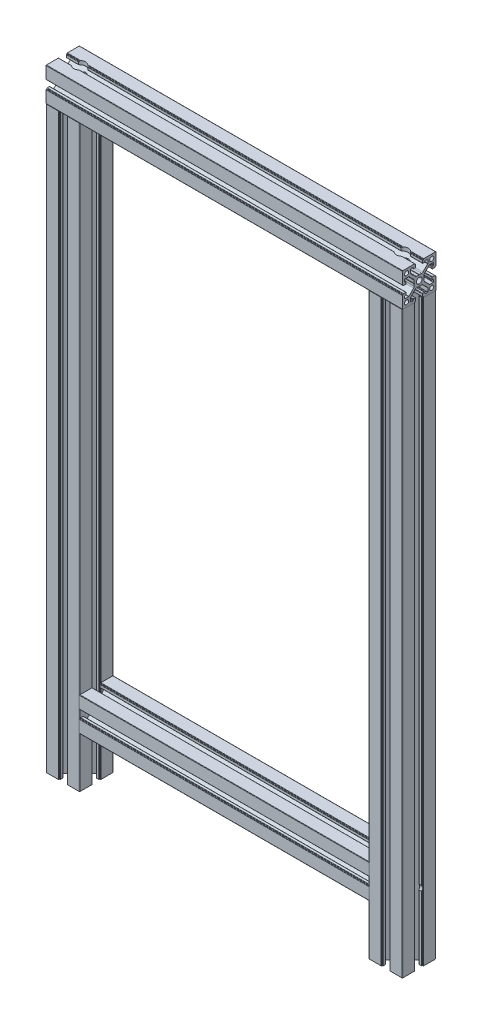
from build123d import *

# Parameters (mm, degrees)
SKETCH_14_R                = 2.45
SKETCH_14_R_2              = 3.4
LE_8_4040HW_DEPTH          = 425
SKETCH_14_ON_SEGMENT_2_R   = 2.45
SKETCH_14_ON_SEGMENT_2_R_2 = 3.4
LE_8_4040HW_2_DEPTH        = 711.5
SKETCH_14_ON_SEGMENT_3_R   = 2.45
SKETCH_14_ON_SEGMENT_3_R_2 = 3.4
LE_8_4040HW_3_DEPTH        = 711.5
SKETCH_14_ON_SEGMENT_4_R   = 2.45
SKETCH_14_ON_SEGMENT_4_R_2 = 3.4
LE_8_4040HW_4_DEPTH        = 387
SKETCH_15_R                = 4.4
CUT_EXTRUDE_1_DEPTH        = 46
SKETCH_16_R                = 5.1
CUT_EXTRUDE_3_DEPTH        = 40
SKETCH_18_R                = 7
CUT_EXTRUDE_8_DEPTH        = 30


with BuildPart() as part:
    # 草图14 → LE-8-4040HW (new body)
    with BuildSketch(Plane(origin=(-212.5, 710.5, 0), x_dir=(0, 1, 0), z_dir=(1, 0, 0))):
        with BuildLine():
            Line((-6, -0.3), (-6, -3.050252532))
            ThreePointArc((-6, -3.050252532), (-6.152240935, -3.815619396), (-6.585786438, -4.464466094))
            Line((-6.585786438, -4.464466094), (-12.224873734, -10.103553391))
            ThreePointArc((-12.224873734, -10.103553391), (-12.387085409, -10.211939766), (-12.578427125, -10.25))
            Line((-12.578427125, -10.25), (-16.8, -10.25))
            ThreePointArc((-16.8, -10.25), (-17.153553391, -10.103553391), (-17.3, -9.75))
            Line((-17.3, -9.75), (-17.3, -7.6))
            ThreePointArc((-17.3, -7.6), (-17.153553391, -7.246446609), (-16.8, -7.1))
            Line((-16.8, -7.1), (-16, -7.1))
            ThreePointArc((-16, -7.1), (-15.646446609, -6.953553391), (-15.5, -6.6))
            Line((-15.5, -6.6), (-15.5, -4.6))
            ThreePointArc((-15.5, -4.6), (-15.646446609, -4.246446609), (-16, -4.1))
            Line((-16, -4.1), (-18.7, -4.1))
            ThreePointArc((-18.7, -4.1), (-18.912132034, -4.187867966), (-19, -4.4))
            Line((-19, -4.4), (-19, -4.8))
            ThreePointArc((-19, -4.8), (-19.087867966, -5.012132034), (-19.3, -5.1))
            Line((-19.3, -5.1), (-19.7, -5.1))
            ThreePointArc((-19.7, -5.1), (-19.912132034, -5.187867966), (-20, -5.4))
            Line((-20, -5.4), (-20, -19.5))
            ThreePointArc((-20, -19.5), (-19.853553391, -19.853553391), (-19.5, -20))
            Line((-19.5, -20), (-5.4, -20))
            ThreePointArc((-5.4, -20), (-5.187867966, -19.912132034), (-5.1, -19.7))
            Line((-5.1, -19.7), (-5.1, -19.3))
            ThreePointArc((-5.1, -19.3), (-5.012132034, -19.087867966), (-4.8, -19))
            Line((-4.8, -19), (-4.4, -19))
            ThreePointArc((-4.4, -19), (-4.187867966, -18.912132034), (-4.1, -18.7))
            Line((-4.1, -18.7), (-4.1, -16))
            ThreePointArc((-4.1, -16), (-4.246446609, -15.646446609), (-4.6, -15.5))
            Line((-4.6, -15.5), (-6.6, -15.5))
            ThreePointArc((-6.6, -15.5), (-6.953553391, -15.646446609), (-7.1, -16))
            Line((-7.1, -16), (-7.1, -16.8))
            ThreePointArc((-7.1, -16.8), (-7.246446609, -17.153553391), (-7.6, -17.3))
            Line((-7.6, -17.3), (-9.75, -17.3))
            ThreePointArc((-9.75, -17.3), (-10.103553391, -17.153553391), (-10.25, -16.8))
            Line((-10.25, -16.8), (-10.25, -12.578427125))
            ThreePointArc((-10.25, -12.578427125), (-10.211939766, -12.387085409), (-10.103553391, -12.224873734))
            Line((-10.103553391, -12.224873734), (-4.464466094, -6.585786438))
            ThreePointArc((-4.464466094, -6.585786438), (-3.815619396, -6.152240935), (-3.050252532, -6))
            Line((-3.050252532, -6), (-0.3, -6))
            ThreePointArc((-0.3, -6), (0, -5.7), (0.3, -6))
            Line((0.3, -6), (3.050252532, -6))
            ThreePointArc((3.050252532, -6), (3.815619396, -6.152240935), (4.464466094, -6.585786438))
            Line((4.464466094, -6.585786438), (10.103553391, -12.224873734))
            ThreePointArc((10.103553391, -12.224873734), (10.211939766, -12.387085409), (10.25, -12.578427125))
            Line((10.25, -12.578427125), (10.25, -16.8))
            ThreePointArc((10.25, -16.8), (10.103553391, -17.153553391), (9.75, -17.3))
            Line((9.75, -17.3), (7.6, -17.3))
            ThreePointArc((7.6, -17.3), (7.246446609, -17.153553391), (7.1, -16.8))
            Line((7.1, -16.8), (7.1, -16))
            ThreePointArc((7.1, -16), (6.953553391, -15.646446609), (6.6, -15.5))
            Line((6.6, -15.5), (4.6, -15.5))
            ThreePointArc((4.6, -15.5), (4.246446609, -15.646446609), (4.1, -16))
            Line((4.1, -16), (4.1, -18.7))
            ThreePointArc((4.1, -18.7), (4.187867966, -18.912132034), (4.4, -19))
            Line((4.4, -19), (4.8, -19))
            ThreePointArc((4.8, -19), (5.012132034, -19.087867966), (5.1, -19.3))
            Line((5.1, -19.3), (5.1, -19.7))
            ThreePointArc((5.1, -19.7), (5.187867966, -19.912132034), (5.4, -20))
            Line((5.4, -20), (19.5, -20))
            ThreePointArc((19.5, -20), (19.853553391, -19.853553391), (20, -19.5))
            Line((20, -19.5), (20, -5.4))
            ThreePointArc((20, -5.4), (19.912132034, -5.187867966), (19.7, -5.1))
            Line((19.7, -5.1), (19.3, -5.1))
            ThreePointArc((19.3, -5.1), (19.087867966, -5.012132034), (19, -4.8))
            Line((19, -4.8), (19, -4.4))
            ThreePointArc((19, -4.4), (18.912132034, -4.187867966), (18.7, -4.1))
            Line((18.7, -4.1), (16, -4.1))
            ThreePointArc((16, -4.1), (15.646446609, -4.246446609), (15.5, -4.6))
            Line((15.5, -4.6), (15.5, -6.6))
            ThreePointArc((15.5, -6.6), (15.646446609, -6.953553391), (16, -7.1))
            Line((16, -7.1), (16.8, -7.1))
            ThreePointArc((16.8, -7.1), (17.153553391, -7.246446609), (17.3, -7.6))
            Line((17.3, -7.6), (17.3, -9.75))
            ThreePointArc((17.3, -9.75), (17.153553391, -10.103553391), (16.8, -10.25))
            Line((16.8, -10.25), (12.578427125, -10.25))
            ThreePointArc((12.578427125, -10.25), (12.387085409, -10.211939766), (12.224873734, -10.103553391))
            Line((12.224873734, -10.103553391), (6.585786438, -4.464466094))
            ThreePointArc((6.585786438, -4.464466094), (6.152240935, -3.815619396), (6, -3.050252532))
            Line((6, -3.050252532), (6, -0.3))
            ThreePointArc((6, -0.3), (5.7, 0), (6, 0.3))
            Line((6, 0.3), (6, 3.050252532))
            ThreePointArc((6, 3.050252532), (6.152240935, 3.815619396), (6.585786438, 4.464466094))
            Line((6.585786438, 4.464466094), (12.224873734, 10.103553391))
            ThreePointArc((12.224873734, 10.103553391), (12.387085409, 10.211939766), (12.578427125, 10.25))
            Line((12.578427125, 10.25), (16.8, 10.25))
            ThreePointArc((16.8, 10.25), (17.153553391, 10.103553391), (17.3, 9.75))
            Line((17.3, 9.75), (17.3, 7.6))
            ThreePointArc((17.3, 7.6), (17.153553391, 7.246446609), (16.8, 7.1))
            Line((16.8, 7.1), (16, 7.1))
            ThreePointArc((16, 7.1), (15.646446609, 6.953553391), (15.5, 6.6))
            Line((15.5, 6.6), (15.5, 4.6))
            ThreePointArc((15.5, 4.6), (15.646446609, 4.246446609), (16, 4.1))
            Line((16, 4.1), (18.7, 4.1))
            ThreePointArc((18.7, 4.1), (18.912132034, 4.187867966), (19, 4.4))
            Line((19, 4.4), (19, 4.8))
            ThreePointArc((19, 4.8), (19.087867966, 5.012132034), (19.3, 5.1))
            Line((19.3, 5.1), (19.7, 5.1))
            ThreePointArc((19.7, 5.1), (19.912132034, 5.187867966), (20, 5.4))
            Line((20, 5.4), (20, 19.5))
            ThreePointArc((20, 19.5), (19.853553391, 19.853553391), (19.5, 20))
            Line((19.5, 20), (5.4, 20))
            ThreePointArc((5.4, 20), (5.187867966, 19.912132034), (5.1, 19.7))
            Line((5.1, 19.7), (5.1, 19.3))
            ThreePointArc((5.1, 19.3), (5.012132034, 19.087867966), (4.8, 19))
            Line((4.8, 19), (4.4, 19))
            ThreePointArc((4.4, 19), (4.187867966, 18.912132034), (4.1, 18.7))
            Line((4.1, 18.7), (4.1, 16))
            ThreePointArc((4.1, 16), (4.246446609, 15.646446609), (4.6, 15.5))
            Line((4.6, 15.5), (6.6, 15.5))
            ThreePointArc((6.6, 15.5), (6.953553391, 15.646446609), (7.1, 16))
            Line((7.1, 16), (7.1, 16.8))
            ThreePointArc((7.1, 16.8), (7.246446609, 17.153553391), (7.6, 17.3))
            Line((7.6, 17.3), (9.75, 17.3))
            ThreePointArc((9.75, 17.3), (10.103553391, 17.153553391), (10.25, 16.8))
            Line((10.25, 16.8), (10.25, 12.578427125))
            ThreePointArc((10.25, 12.578427125), (10.211939766, 12.387085409), (10.103553391, 12.224873734))
            Line((10.103553391, 12.224873734), (4.464466094, 6.585786438))
            ThreePointArc((4.464466094, 6.585786438), (3.815619396, 6.152240935), (3.050252532, 6))
            Line((3.050252532, 6), (0.3, 6))
            ThreePointArc((0.3, 6), (0, 5.7), (-0.3, 6))
            Line((-0.3, 6), (-3.050252532, 6))
            ThreePointArc((-3.050252532, 6), (-3.815619396, 6.152240935), (-4.464466094, 6.585786438))
            Line((-4.464466094, 6.585786438), (-10.103553391, 12.224873734))
            ThreePointArc((-10.103553391, 12.224873734), (-10.211939766, 12.387085409), (-10.25, 12.578427125))
            Line((-10.25, 12.578427125), (-10.25, 16.8))
            ThreePointArc((-10.25, 16.8), (-10.103553391, 17.153553391), (-9.75, 17.3))
            Line((-9.75, 17.3), (-7.6, 17.3))
            ThreePointArc((-7.6, 17.3), (-7.246446609, 17.153553391), (-7.1, 16.8))
            Line((-7.1, 16.8), (-7.1, 16))
            ThreePointArc((-7.1, 16), (-6.953553391, 15.646446609), (-6.6, 15.5))
            Line((-6.6, 15.5), (-4.6, 15.5))
            ThreePointArc((-4.6, 15.5), (-4.246446609, 15.646446609), (-4.1, 16))
            Line((-4.1, 16), (-4.1, 18.7))
            ThreePointArc((-4.1, 18.7), (-4.187867966, 18.912132034), (-4.4, 19))
            Line((-4.4, 19), (-4.8, 19))
            ThreePointArc((-4.8, 19), (-5.012132034, 19.087867966), (-5.1, 19.3))
            Line((-5.1, 19.3), (-5.1, 19.7))
            ThreePointArc((-5.1, 19.7), (-5.187867966, 19.912132034), (-5.4, 20))
            Line((-5.4, 20), (-19.5, 20))
            ThreePointArc((-19.5, 20), (-19.853553391, 19.853553391), (-20, 19.5))
            Line((-20, 19.5), (-20, 5.4))
            ThreePointArc((-20, 5.4), (-19.912132034, 5.187867966), (-19.7, 5.1))
            Line((-19.7, 5.1), (-19.3, 5.1))
            ThreePointArc((-19.3, 5.1), (-19.087867966, 5.012132034), (-19, 4.8))
            Line((-19, 4.8), (-19, 4.4))
            ThreePointArc((-19, 4.4), (-18.912132034, 4.187867966), (-18.7, 4.1))
            Line((-18.7, 4.1), (-16, 4.1))
            ThreePointArc((-16, 4.1), (-15.646446609, 4.246446609), (-15.5, 4.6))
            Line((-15.5, 4.6), (-15.5, 6.6))
            ThreePointArc((-15.5, 6.6), (-15.646446609, 6.953553391), (-16, 7.1))
            Line((-16, 7.1), (-16.8, 7.1))
            ThreePointArc((-16.8, 7.1), (-17.153553391, 7.246446609), (-17.3, 7.6))
            Line((-17.3, 7.6), (-17.3, 9.75))
            ThreePointArc((-17.3, 9.75), (-17.153553391, 10.103553391), (-16.8, 10.25))
            Line((-16.8, 10.25), (-12.578427125, 10.25))
            ThreePointArc((-12.578427125, 10.25), (-12.387085409, 10.211939766), (-12.224873734, 10.103553391))
            Line((-12.224873734, 10.103553391), (-6.585786438, 4.464466094))
            ThreePointArc((-6.585786438, 4.464466094), (-6.152240935, 3.815619396), (-6, 3.050252532))
            Line((-6, 3.050252532), (-6, 0.3))
            ThreePointArc((-6, 0.3), (-5.7, 0), (-6, -0.3))
        make_face()
        with Locations((-15, 15)):
            Circle(SKETCH_14_R, mode=Mode.SUBTRACT)
        Circle(SKETCH_14_R_2, mode=Mode.SUBTRACT)
        with Locations((15, 15)):
            Circle(SKETCH_14_R, mode=Mode.SUBTRACT)
        with Locations((15, -15)):
            Circle(SKETCH_14_R, mode=Mode.SUBTRACT)
        with Locations((-15, -15)):
            Circle(SKETCH_14_R, mode=Mode.SUBTRACT)
    extrude(amount=LE_8_4040HW_DEPTH)

    # 草图18 → 切除-拉伸8 (cut)
    with BuildSketch(Plane(origin=(0, 730.5, 0), x_dir=(1, 0, 0), z_dir=(0, 1, 0))):
        with Locations(Location((192.5, 0, 0), (0, 0, 320.373457062))):
            Circle(SKETCH_18_R)
        with Locations(Location((-192.5, 0, 0), (0, 0, 320.373457062))):
            Circle(SKETCH_18_R)
    extrude(amount=-CUT_EXTRUDE_8_DEPTH, mode=Mode.SUBTRACT)


with BuildPart() as body_2:
    # 草图14 on segment 2 (carried to segment 2) → LE-8-4040HW 2 (new body)
    with BuildSketch(Plane(origin=(-192.5, 0, 0), x_dir=(-1, 0, 0), z_dir=(0, 1, 0))):
        with BuildLine():
            Line((-6, -0.3), (-6, -3.050252532))
            ThreePointArc((-6, -3.050252532), (-6.152240935, -3.815619396), (-6.585786438, -4.464466094))
            Line((-6.585786438, -4.464466094), (-12.224873734, -10.103553391))
            ThreePointArc((-12.224873734, -10.103553391), (-12.387085409, -10.211939766), (-12.578427125, -10.25))
            Line((-12.578427125, -10.25), (-16.8, -10.25))
            ThreePointArc((-16.8, -10.25), (-17.153553391, -10.103553391), (-17.3, -9.75))
            Line((-17.3, -9.75), (-17.3, -7.6))
            ThreePointArc((-17.3, -7.6), (-17.153553391, -7.246446609), (-16.8, -7.1))
            Line((-16.8, -7.1), (-16, -7.1))
            ThreePointArc((-16, -7.1), (-15.646446609, -6.953553391), (-15.5, -6.6))
            Line((-15.5, -6.6), (-15.5, -4.6))
            ThreePointArc((-15.5, -4.6), (-15.646446609, -4.246446609), (-16, -4.1))
            Line((-16, -4.1), (-18.7, -4.1))
            ThreePointArc((-18.7, -4.1), (-18.912132034, -4.187867966), (-19, -4.4))
            Line((-19, -4.4), (-19, -4.8))
            ThreePointArc((-19, -4.8), (-19.087867966, -5.012132034), (-19.3, -5.1))
            Line((-19.3, -5.1), (-19.7, -5.1))
            ThreePointArc((-19.7, -5.1), (-19.912132034, -5.187867966), (-20, -5.4))
            Line((-20, -5.4), (-20, -19.5))
            ThreePointArc((-20, -19.5), (-19.853553391, -19.853553391), (-19.5, -20))
            Line((-19.5, -20), (-5.4, -20))
            ThreePointArc((-5.4, -20), (-5.187867966, -19.912132034), (-5.1, -19.7))
            Line((-5.1, -19.7), (-5.1, -19.3))
            ThreePointArc((-5.1, -19.3), (-5.012132034, -19.087867966), (-4.8, -19))
            Line((-4.8, -19), (-4.4, -19))
            ThreePointArc((-4.4, -19), (-4.187867966, -18.912132034), (-4.1, -18.7))
            Line((-4.1, -18.7), (-4.1, -16))
            ThreePointArc((-4.1, -16), (-4.246446609, -15.646446609), (-4.6, -15.5))
            Line((-4.6, -15.5), (-6.6, -15.5))
            ThreePointArc((-6.6, -15.5), (-6.953553391, -15.646446609), (-7.1, -16))
            Line((-7.1, -16), (-7.1, -16.8))
            ThreePointArc((-7.1, -16.8), (-7.246446609, -17.153553391), (-7.6, -17.3))
            Line((-7.6, -17.3), (-9.75, -17.3))
            ThreePointArc((-9.75, -17.3), (-10.103553391, -17.153553391), (-10.25, -16.8))
            Line((-10.25, -16.8), (-10.25, -12.578427125))
            ThreePointArc((-10.25, -12.578427125), (-10.211939766, -12.387085409), (-10.103553391, -12.224873734))
            Line((-10.103553391, -12.224873734), (-4.464466094, -6.585786438))
            ThreePointArc((-4.464466094, -6.585786438), (-3.815619396, -6.152240935), (-3.050252532, -6))
            Line((-3.050252532, -6), (-0.3, -6))
            ThreePointArc((-0.3, -6), (0, -5.7), (0.3, -6))
            Line((0.3, -6), (3.050252532, -6))
            ThreePointArc((3.050252532, -6), (3.815619396, -6.152240935), (4.464466094, -6.585786438))
            Line((4.464466094, -6.585786438), (10.103553391, -12.224873734))
            ThreePointArc((10.103553391, -12.224873734), (10.211939766, -12.387085409), (10.25, -12.578427125))
            Line((10.25, -12.578427125), (10.25, -16.8))
            ThreePointArc((10.25, -16.8), (10.103553391, -17.153553391), (9.75, -17.3))
            Line((9.75, -17.3), (7.6, -17.3))
            ThreePointArc((7.6, -17.3), (7.246446609, -17.153553391), (7.1, -16.8))
            Line((7.1, -16.8), (7.1, -16))
            ThreePointArc((7.1, -16), (6.953553391, -15.646446609), (6.6, -15.5))
            Line((6.6, -15.5), (4.6, -15.5))
            ThreePointArc((4.6, -15.5), (4.246446609, -15.646446609), (4.1, -16))
            Line((4.1, -16), (4.1, -18.7))
            ThreePointArc((4.1, -18.7), (4.187867966, -18.912132034), (4.4, -19))
            Line((4.4, -19), (4.8, -19))
            ThreePointArc((4.8, -19), (5.012132034, -19.087867966), (5.1, -19.3))
            Line((5.1, -19.3), (5.1, -19.7))
            ThreePointArc((5.1, -19.7), (5.187867966, -19.912132034), (5.4, -20))
            Line((5.4, -20), (19.5, -20))
            ThreePointArc((19.5, -20), (19.853553391, -19.853553391), (20, -19.5))
            Line((20, -19.5), (20, -5.4))
            ThreePointArc((20, -5.4), (19.912132034, -5.187867966), (19.7, -5.1))
            Line((19.7, -5.1), (19.3, -5.1))
            ThreePointArc((19.3, -5.1), (19.087867966, -5.012132034), (19, -4.8))
            Line((19, -4.8), (19, -4.4))
            ThreePointArc((19, -4.4), (18.912132034, -4.187867966), (18.7, -4.1))
            Line((18.7, -4.1), (16, -4.1))
            ThreePointArc((16, -4.1), (15.646446609, -4.246446609), (15.5, -4.6))
            Line((15.5, -4.6), (15.5, -6.6))
            ThreePointArc((15.5, -6.6), (15.646446609, -6.953553391), (16, -7.1))
            Line((16, -7.1), (16.8, -7.1))
            ThreePointArc((16.8, -7.1), (17.153553391, -7.246446609), (17.3, -7.6))
            Line((17.3, -7.6), (17.3, -9.75))
            ThreePointArc((17.3, -9.75), (17.153553391, -10.103553391), (16.8, -10.25))
            Line((16.8, -10.25), (12.578427125, -10.25))
            ThreePointArc((12.578427125, -10.25), (12.387085409, -10.211939766), (12.224873734, -10.103553391))
            Line((12.224873734, -10.103553391), (6.585786438, -4.464466094))
            ThreePointArc((6.585786438, -4.464466094), (6.152240935, -3.815619396), (6, -3.050252532))
            Line((6, -3.050252532), (6, -0.3))
            ThreePointArc((6, -0.3), (5.7, 0), (6, 0.3))
            Line((6, 0.3), (6, 3.050252532))
            ThreePointArc((6, 3.050252532), (6.152240935, 3.815619396), (6.585786438, 4.464466094))
            Line((6.585786438, 4.464466094), (12.224873734, 10.103553391))
            ThreePointArc((12.224873734, 10.103553391), (12.387085409, 10.211939766), (12.578427125, 10.25))
            Line((12.578427125, 10.25), (16.8, 10.25))
            ThreePointArc((16.8, 10.25), (17.153553391, 10.103553391), (17.3, 9.75))
            Line((17.3, 9.75), (17.3, 7.6))
            ThreePointArc((17.3, 7.6), (17.153553391, 7.246446609), (16.8, 7.1))
            Line((16.8, 7.1), (16, 7.1))
            ThreePointArc((16, 7.1), (15.646446609, 6.953553391), (15.5, 6.6))
            Line((15.5, 6.6), (15.5, 4.6))
            ThreePointArc((15.5, 4.6), (15.646446609, 4.246446609), (16, 4.1))
            Line((16, 4.1), (18.7, 4.1))
            ThreePointArc((18.7, 4.1), (18.912132034, 4.187867966), (19, 4.4))
            Line((19, 4.4), (19, 4.8))
            ThreePointArc((19, 4.8), (19.087867966, 5.012132034), (19.3, 5.1))
            Line((19.3, 5.1), (19.7, 5.1))
            ThreePointArc((19.7, 5.1), (19.912132034, 5.187867966), (20, 5.4))
            Line((20, 5.4), (20, 19.5))
            ThreePointArc((20, 19.5), (19.853553391, 19.853553391), (19.5, 20))
            Line((19.5, 20), (5.4, 20))
            ThreePointArc((5.4, 20), (5.187867966, 19.912132034), (5.1, 19.7))
            Line((5.1, 19.7), (5.1, 19.3))
            ThreePointArc((5.1, 19.3), (5.012132034, 19.087867966), (4.8, 19))
            Line((4.8, 19), (4.4, 19))
            ThreePointArc((4.4, 19), (4.187867966, 18.912132034), (4.1, 18.7))
            Line((4.1, 18.7), (4.1, 16))
            ThreePointArc((4.1, 16), (4.246446609, 15.646446609), (4.6, 15.5))
            Line((4.6, 15.5), (6.6, 15.5))
            ThreePointArc((6.6, 15.5), (6.953553391, 15.646446609), (7.1, 16))
            Line((7.1, 16), (7.1, 16.8))
            ThreePointArc((7.1, 16.8), (7.246446609, 17.153553391), (7.6, 17.3))
            Line((7.6, 17.3), (9.75, 17.3))
            ThreePointArc((9.75, 17.3), (10.103553391, 17.153553391), (10.25, 16.8))
            Line((10.25, 16.8), (10.25, 12.578427125))
            ThreePointArc((10.25, 12.578427125), (10.211939766, 12.387085409), (10.103553391, 12.224873734))
            Line((10.103553391, 12.224873734), (4.464466094, 6.585786438))
            ThreePointArc((4.464466094, 6.585786438), (3.815619396, 6.152240935), (3.050252532, 6))
            Line((3.050252532, 6), (0.3, 6))
            ThreePointArc((0.3, 6), (0, 5.7), (-0.3, 6))
            Line((-0.3, 6), (-3.050252532, 6))
            ThreePointArc((-3.050252532, 6), (-3.815619396, 6.152240935), (-4.464466094, 6.585786438))
            Line((-4.464466094, 6.585786438), (-10.103553391, 12.224873734))
            ThreePointArc((-10.103553391, 12.224873734), (-10.211939766, 12.387085409), (-10.25, 12.578427125))
            Line((-10.25, 12.578427125), (-10.25, 16.8))
            ThreePointArc((-10.25, 16.8), (-10.103553391, 17.153553391), (-9.75, 17.3))
            Line((-9.75, 17.3), (-7.6, 17.3))
            ThreePointArc((-7.6, 17.3), (-7.246446609, 17.153553391), (-7.1, 16.8))
            Line((-7.1, 16.8), (-7.1, 16))
            ThreePointArc((-7.1, 16), (-6.953553391, 15.646446609), (-6.6, 15.5))
            Line((-6.6, 15.5), (-4.6, 15.5))
            ThreePointArc((-4.6, 15.5), (-4.246446609, 15.646446609), (-4.1, 16))
            Line((-4.1, 16), (-4.1, 18.7))
            ThreePointArc((-4.1, 18.7), (-4.187867966, 18.912132034), (-4.4, 19))
            Line((-4.4, 19), (-4.8, 19))
            ThreePointArc((-4.8, 19), (-5.012132034, 19.087867966), (-5.1, 19.3))
            Line((-5.1, 19.3), (-5.1, 19.7))
            ThreePointArc((-5.1, 19.7), (-5.187867966, 19.912132034), (-5.4, 20))
            Line((-5.4, 20), (-19.5, 20))
            ThreePointArc((-19.5, 20), (-19.853553391, 19.853553391), (-20, 19.5))
            Line((-20, 19.5), (-20, 5.4))
            ThreePointArc((-20, 5.4), (-19.912132034, 5.187867966), (-19.7, 5.1))
            Line((-19.7, 5.1), (-19.3, 5.1))
            ThreePointArc((-19.3, 5.1), (-19.087867966, 5.012132034), (-19, 4.8))
            Line((-19, 4.8), (-19, 4.4))
            ThreePointArc((-19, 4.4), (-18.912132034, 4.187867966), (-18.7, 4.1))
            Line((-18.7, 4.1), (-16, 4.1))
            ThreePointArc((-16, 4.1), (-15.646446609, 4.246446609), (-15.5, 4.6))
            Line((-15.5, 4.6), (-15.5, 6.6))
            ThreePointArc((-15.5, 6.6), (-15.646446609, 6.953553391), (-16, 7.1))
            Line((-16, 7.1), (-16.8, 7.1))
            ThreePointArc((-16.8, 7.1), (-17.153553391, 7.246446609), (-17.3, 7.6))
            Line((-17.3, 7.6), (-17.3, 9.75))
            ThreePointArc((-17.3, 9.75), (-17.153553391, 10.103553391), (-16.8, 10.25))
            Line((-16.8, 10.25), (-12.578427125, 10.25))
            ThreePointArc((-12.578427125, 10.25), (-12.387085409, 10.211939766), (-12.224873734, 10.103553391))
            Line((-12.224873734, 10.103553391), (-6.585786438, 4.464466094))
            ThreePointArc((-6.585786438, 4.464466094), (-6.152240935, 3.815619396), (-6, 3.050252532))
            Line((-6, 3.050252532), (-6, 0.3))
            ThreePointArc((-6, 0.3), (-5.7, 0), (-6, -0.3))
        make_face()
        with Locations((-15, 15)):
            Circle(SKETCH_14_ON_SEGMENT_2_R, mode=Mode.SUBTRACT)
        Circle(SKETCH_14_ON_SEGMENT_2_R_2, mode=Mode.SUBTRACT)
        with Locations((15, 15)):
            Circle(SKETCH_14_ON_SEGMENT_2_R, mode=Mode.SUBTRACT)
        with Locations((15, -15)):
            Circle(SKETCH_14_ON_SEGMENT_2_R, mode=Mode.SUBTRACT)
        with Locations((-15, -15)):
            Circle(SKETCH_14_ON_SEGMENT_2_R, mode=Mode.SUBTRACT)
    extrude(amount=LE_8_4040HW_2_DEPTH)

    # LE-8-4040HW 2 end butt 1
    split(bisect_by=Plane(origin=(-192.5, 690.5, 0), x_dir=(1, 0, 0), z_dir=(0, -1, 0)), keep=Keep.TOP)


with BuildPart() as body_3:
    # 草图14 on segment 3 (carried to segment 3) → LE-8-4040HW 3 (new body)
    with BuildSketch(Plane(origin=(192.5, 0, 0), x_dir=(-1, 0, 0), z_dir=(0, 1, 0))):
        with BuildLine():
            Line((-6, -0.3), (-6, -3.050252532))
            ThreePointArc((-6, -3.050252532), (-6.152240935, -3.815619396), (-6.585786438, -4.464466094))
            Line((-6.585786438, -4.464466094), (-12.224873734, -10.103553391))
            ThreePointArc((-12.224873734, -10.103553391), (-12.387085409, -10.211939766), (-12.578427125, -10.25))
            Line((-12.578427125, -10.25), (-16.8, -10.25))
            ThreePointArc((-16.8, -10.25), (-17.153553391, -10.103553391), (-17.3, -9.75))
            Line((-17.3, -9.75), (-17.3, -7.6))
            ThreePointArc((-17.3, -7.6), (-17.153553391, -7.246446609), (-16.8, -7.1))
            Line((-16.8, -7.1), (-16, -7.1))
            ThreePointArc((-16, -7.1), (-15.646446609, -6.953553391), (-15.5, -6.6))
            Line((-15.5, -6.6), (-15.5, -4.6))
            ThreePointArc((-15.5, -4.6), (-15.646446609, -4.246446609), (-16, -4.1))
            Line((-16, -4.1), (-18.7, -4.1))
            ThreePointArc((-18.7, -4.1), (-18.912132034, -4.187867966), (-19, -4.4))
            Line((-19, -4.4), (-19, -4.8))
            ThreePointArc((-19, -4.8), (-19.087867966, -5.012132034), (-19.3, -5.1))
            Line((-19.3, -5.1), (-19.7, -5.1))
            ThreePointArc((-19.7, -5.1), (-19.912132034, -5.187867966), (-20, -5.4))
            Line((-20, -5.4), (-20, -19.5))
            ThreePointArc((-20, -19.5), (-19.853553391, -19.853553391), (-19.5, -20))
            Line((-19.5, -20), (-5.4, -20))
            ThreePointArc((-5.4, -20), (-5.187867966, -19.912132034), (-5.1, -19.7))
            Line((-5.1, -19.7), (-5.1, -19.3))
            ThreePointArc((-5.1, -19.3), (-5.012132034, -19.087867966), (-4.8, -19))
            Line((-4.8, -19), (-4.4, -19))
            ThreePointArc((-4.4, -19), (-4.187867966, -18.912132034), (-4.1, -18.7))
            Line((-4.1, -18.7), (-4.1, -16))
            ThreePointArc((-4.1, -16), (-4.246446609, -15.646446609), (-4.6, -15.5))
            Line((-4.6, -15.5), (-6.6, -15.5))
            ThreePointArc((-6.6, -15.5), (-6.953553391, -15.646446609), (-7.1, -16))
            Line((-7.1, -16), (-7.1, -16.8))
            ThreePointArc((-7.1, -16.8), (-7.246446609, -17.153553391), (-7.6, -17.3))
            Line((-7.6, -17.3), (-9.75, -17.3))
            ThreePointArc((-9.75, -17.3), (-10.103553391, -17.153553391), (-10.25, -16.8))
            Line((-10.25, -16.8), (-10.25, -12.578427125))
            ThreePointArc((-10.25, -12.578427125), (-10.211939766, -12.387085409), (-10.103553391, -12.224873734))
            Line((-10.103553391, -12.224873734), (-4.464466094, -6.585786438))
            ThreePointArc((-4.464466094, -6.585786438), (-3.815619396, -6.152240935), (-3.050252532, -6))
            Line((-3.050252532, -6), (-0.3, -6))
            ThreePointArc((-0.3, -6), (0, -5.7), (0.3, -6))
            Line((0.3, -6), (3.050252532, -6))
            ThreePointArc((3.050252532, -6), (3.815619396, -6.152240935), (4.464466094, -6.585786438))
            Line((4.464466094, -6.585786438), (10.103553391, -12.224873734))
            ThreePointArc((10.103553391, -12.224873734), (10.211939766, -12.387085409), (10.25, -12.578427125))
            Line((10.25, -12.578427125), (10.25, -16.8))
            ThreePointArc((10.25, -16.8), (10.103553391, -17.153553391), (9.75, -17.3))
            Line((9.75, -17.3), (7.6, -17.3))
            ThreePointArc((7.6, -17.3), (7.246446609, -17.153553391), (7.1, -16.8))
            Line((7.1, -16.8), (7.1, -16))
            ThreePointArc((7.1, -16), (6.953553391, -15.646446609), (6.6, -15.5))
            Line((6.6, -15.5), (4.6, -15.5))
            ThreePointArc((4.6, -15.5), (4.246446609, -15.646446609), (4.1, -16))
            Line((4.1, -16), (4.1, -18.7))
            ThreePointArc((4.1, -18.7), (4.187867966, -18.912132034), (4.4, -19))
            Line((4.4, -19), (4.8, -19))
            ThreePointArc((4.8, -19), (5.012132034, -19.087867966), (5.1, -19.3))
            Line((5.1, -19.3), (5.1, -19.7))
            ThreePointArc((5.1, -19.7), (5.187867966, -19.912132034), (5.4, -20))
            Line((5.4, -20), (19.5, -20))
            ThreePointArc((19.5, -20), (19.853553391, -19.853553391), (20, -19.5))
            Line((20, -19.5), (20, -5.4))
            ThreePointArc((20, -5.4), (19.912132034, -5.187867966), (19.7, -5.1))
            Line((19.7, -5.1), (19.3, -5.1))
            ThreePointArc((19.3, -5.1), (19.087867966, -5.012132034), (19, -4.8))
            Line((19, -4.8), (19, -4.4))
            ThreePointArc((19, -4.4), (18.912132034, -4.187867966), (18.7, -4.1))
            Line((18.7, -4.1), (16, -4.1))
            ThreePointArc((16, -4.1), (15.646446609, -4.246446609), (15.5, -4.6))
            Line((15.5, -4.6), (15.5, -6.6))
            ThreePointArc((15.5, -6.6), (15.646446609, -6.953553391), (16, -7.1))
            Line((16, -7.1), (16.8, -7.1))
            ThreePointArc((16.8, -7.1), (17.153553391, -7.246446609), (17.3, -7.6))
            Line((17.3, -7.6), (17.3, -9.75))
            ThreePointArc((17.3, -9.75), (17.153553391, -10.103553391), (16.8, -10.25))
            Line((16.8, -10.25), (12.578427125, -10.25))
            ThreePointArc((12.578427125, -10.25), (12.387085409, -10.211939766), (12.224873734, -10.103553391))
            Line((12.224873734, -10.103553391), (6.585786438, -4.464466094))
            ThreePointArc((6.585786438, -4.464466094), (6.152240935, -3.815619396), (6, -3.050252532))
            Line((6, -3.050252532), (6, -0.3))
            ThreePointArc((6, -0.3), (5.7, 0), (6, 0.3))
            Line((6, 0.3), (6, 3.050252532))
            ThreePointArc((6, 3.050252532), (6.152240935, 3.815619396), (6.585786438, 4.464466094))
            Line((6.585786438, 4.464466094), (12.224873734, 10.103553391))
            ThreePointArc((12.224873734, 10.103553391), (12.387085409, 10.211939766), (12.578427125, 10.25))
            Line((12.578427125, 10.25), (16.8, 10.25))
            ThreePointArc((16.8, 10.25), (17.153553391, 10.103553391), (17.3, 9.75))
            Line((17.3, 9.75), (17.3, 7.6))
            ThreePointArc((17.3, 7.6), (17.153553391, 7.246446609), (16.8, 7.1))
            Line((16.8, 7.1), (16, 7.1))
            ThreePointArc((16, 7.1), (15.646446609, 6.953553391), (15.5, 6.6))
            Line((15.5, 6.6), (15.5, 4.6))
            ThreePointArc((15.5, 4.6), (15.646446609, 4.246446609), (16, 4.1))
            Line((16, 4.1), (18.7, 4.1))
            ThreePointArc((18.7, 4.1), (18.912132034, 4.187867966), (19, 4.4))
            Line((19, 4.4), (19, 4.8))
            ThreePointArc((19, 4.8), (19.087867966, 5.012132034), (19.3, 5.1))
            Line((19.3, 5.1), (19.7, 5.1))
            ThreePointArc((19.7, 5.1), (19.912132034, 5.187867966), (20, 5.4))
            Line((20, 5.4), (20, 19.5))
            ThreePointArc((20, 19.5), (19.853553391, 19.853553391), (19.5, 20))
            Line((19.5, 20), (5.4, 20))
            ThreePointArc((5.4, 20), (5.187867966, 19.912132034), (5.1, 19.7))
            Line((5.1, 19.7), (5.1, 19.3))
            ThreePointArc((5.1, 19.3), (5.012132034, 19.087867966), (4.8, 19))
            Line((4.8, 19), (4.4, 19))
            ThreePointArc((4.4, 19), (4.187867966, 18.912132034), (4.1, 18.7))
            Line((4.1, 18.7), (4.1, 16))
            ThreePointArc((4.1, 16), (4.246446609, 15.646446609), (4.6, 15.5))
            Line((4.6, 15.5), (6.6, 15.5))
            ThreePointArc((6.6, 15.5), (6.953553391, 15.646446609), (7.1, 16))
            Line((7.1, 16), (7.1, 16.8))
            ThreePointArc((7.1, 16.8), (7.246446609, 17.153553391), (7.6, 17.3))
            Line((7.6, 17.3), (9.75, 17.3))
            ThreePointArc((9.75, 17.3), (10.103553391, 17.153553391), (10.25, 16.8))
            Line((10.25, 16.8), (10.25, 12.578427125))
            ThreePointArc((10.25, 12.578427125), (10.211939766, 12.387085409), (10.103553391, 12.224873734))
            Line((10.103553391, 12.224873734), (4.464466094, 6.585786438))
            ThreePointArc((4.464466094, 6.585786438), (3.815619396, 6.152240935), (3.050252532, 6))
            Line((3.050252532, 6), (0.3, 6))
            ThreePointArc((0.3, 6), (0, 5.7), (-0.3, 6))
            Line((-0.3, 6), (-3.050252532, 6))
            ThreePointArc((-3.050252532, 6), (-3.815619396, 6.152240935), (-4.464466094, 6.585786438))
            Line((-4.464466094, 6.585786438), (-10.103553391, 12.224873734))
            ThreePointArc((-10.103553391, 12.224873734), (-10.211939766, 12.387085409), (-10.25, 12.578427125))
            Line((-10.25, 12.578427125), (-10.25, 16.8))
            ThreePointArc((-10.25, 16.8), (-10.103553391, 17.153553391), (-9.75, 17.3))
            Line((-9.75, 17.3), (-7.6, 17.3))
            ThreePointArc((-7.6, 17.3), (-7.246446609, 17.153553391), (-7.1, 16.8))
            Line((-7.1, 16.8), (-7.1, 16))
            ThreePointArc((-7.1, 16), (-6.953553391, 15.646446609), (-6.6, 15.5))
            Line((-6.6, 15.5), (-4.6, 15.5))
            ThreePointArc((-4.6, 15.5), (-4.246446609, 15.646446609), (-4.1, 16))
            Line((-4.1, 16), (-4.1, 18.7))
            ThreePointArc((-4.1, 18.7), (-4.187867966, 18.912132034), (-4.4, 19))
            Line((-4.4, 19), (-4.8, 19))
            ThreePointArc((-4.8, 19), (-5.012132034, 19.087867966), (-5.1, 19.3))
            Line((-5.1, 19.3), (-5.1, 19.7))
            ThreePointArc((-5.1, 19.7), (-5.187867966, 19.912132034), (-5.4, 20))
            Line((-5.4, 20), (-19.5, 20))
            ThreePointArc((-19.5, 20), (-19.853553391, 19.853553391), (-20, 19.5))
            Line((-20, 19.5), (-20, 5.4))
            ThreePointArc((-20, 5.4), (-19.912132034, 5.187867966), (-19.7, 5.1))
            Line((-19.7, 5.1), (-19.3, 5.1))
            ThreePointArc((-19.3, 5.1), (-19.087867966, 5.012132034), (-19, 4.8))
            Line((-19, 4.8), (-19, 4.4))
            ThreePointArc((-19, 4.4), (-18.912132034, 4.187867966), (-18.7, 4.1))
            Line((-18.7, 4.1), (-16, 4.1))
            ThreePointArc((-16, 4.1), (-15.646446609, 4.246446609), (-15.5, 4.6))
            Line((-15.5, 4.6), (-15.5, 6.6))
            ThreePointArc((-15.5, 6.6), (-15.646446609, 6.953553391), (-16, 7.1))
            Line((-16, 7.1), (-16.8, 7.1))
            ThreePointArc((-16.8, 7.1), (-17.153553391, 7.246446609), (-17.3, 7.6))
            Line((-17.3, 7.6), (-17.3, 9.75))
            ThreePointArc((-17.3, 9.75), (-17.153553391, 10.103553391), (-16.8, 10.25))
            Line((-16.8, 10.25), (-12.578427125, 10.25))
            ThreePointArc((-12.578427125, 10.25), (-12.387085409, 10.211939766), (-12.224873734, 10.103553391))
            Line((-12.224873734, 10.103553391), (-6.585786438, 4.464466094))
            ThreePointArc((-6.585786438, 4.464466094), (-6.152240935, 3.815619396), (-6, 3.050252532))
            Line((-6, 3.050252532), (-6, 0.3))
            ThreePointArc((-6, 0.3), (-5.7, 0), (-6, -0.3))
        make_face()
        with Locations((-15, 15)):
            Circle(SKETCH_14_ON_SEGMENT_3_R, mode=Mode.SUBTRACT)
        Circle(SKETCH_14_ON_SEGMENT_3_R_2, mode=Mode.SUBTRACT)
        with Locations((15, 15)):
            Circle(SKETCH_14_ON_SEGMENT_3_R, mode=Mode.SUBTRACT)
        with Locations((15, -15)):
            Circle(SKETCH_14_ON_SEGMENT_3_R, mode=Mode.SUBTRACT)
        with Locations((-15, -15)):
            Circle(SKETCH_14_ON_SEGMENT_3_R, mode=Mode.SUBTRACT)
    extrude(amount=LE_8_4040HW_3_DEPTH)

    # LE-8-4040HW 3 end butt 1
    split(bisect_by=Plane(origin=(192.5, 690.5, 0), x_dir=(1, 0, 0), z_dir=(0, -1, 0)), keep=Keep.TOP)

    # 草图16 → 切除-拉伸3 (cut)
    with BuildSketch(Plane(origin=(212.5, 0, 0), x_dir=(0, 0, -1), z_dir=(1, 0, 0))):
        with Locations(Location((0, 80, 0), (0, 0, 28.909366673))):
            Circle(SKETCH_16_R)
    extrude(amount=-CUT_EXTRUDE_3_DEPTH, mode=Mode.SUBTRACT)


with BuildPart() as body_4:
    # 草图14 on segment 4 (carried to segment 4) → LE-8-4040HW 4 (new body)
    with BuildSketch(Plane(origin=(-193.5, 80, 0), x_dir=(0, 1, 0), z_dir=(1, 0, 0))):
        with BuildLine():
            Line((-6, -0.3), (-6, -3.050252532))
            ThreePointArc((-6, -3.050252532), (-6.152240935, -3.815619396), (-6.585786438, -4.464466094))
            Line((-6.585786438, -4.464466094), (-12.224873734, -10.103553391))
            ThreePointArc((-12.224873734, -10.103553391), (-12.387085409, -10.211939766), (-12.578427125, -10.25))
            Line((-12.578427125, -10.25), (-16.8, -10.25))
            ThreePointArc((-16.8, -10.25), (-17.153553391, -10.103553391), (-17.3, -9.75))
            Line((-17.3, -9.75), (-17.3, -7.6))
            ThreePointArc((-17.3, -7.6), (-17.153553391, -7.246446609), (-16.8, -7.1))
            Line((-16.8, -7.1), (-16, -7.1))
            ThreePointArc((-16, -7.1), (-15.646446609, -6.953553391), (-15.5, -6.6))
            Line((-15.5, -6.6), (-15.5, -4.6))
            ThreePointArc((-15.5, -4.6), (-15.646446609, -4.246446609), (-16, -4.1))
            Line((-16, -4.1), (-18.7, -4.1))
            ThreePointArc((-18.7, -4.1), (-18.912132034, -4.187867966), (-19, -4.4))
            Line((-19, -4.4), (-19, -4.8))
            ThreePointArc((-19, -4.8), (-19.087867966, -5.012132034), (-19.3, -5.1))
            Line((-19.3, -5.1), (-19.7, -5.1))
            ThreePointArc((-19.7, -5.1), (-19.912132034, -5.187867966), (-20, -5.4))
            Line((-20, -5.4), (-20, -19.5))
            ThreePointArc((-20, -19.5), (-19.853553391, -19.853553391), (-19.5, -20))
            Line((-19.5, -20), (-5.4, -20))
            ThreePointArc((-5.4, -20), (-5.187867966, -19.912132034), (-5.1, -19.7))
            Line((-5.1, -19.7), (-5.1, -19.3))
            ThreePointArc((-5.1, -19.3), (-5.012132034, -19.087867966), (-4.8, -19))
            Line((-4.8, -19), (-4.4, -19))
            ThreePointArc((-4.4, -19), (-4.187867966, -18.912132034), (-4.1, -18.7))
            Line((-4.1, -18.7), (-4.1, -16))
            ThreePointArc((-4.1, -16), (-4.246446609, -15.646446609), (-4.6, -15.5))
            Line((-4.6, -15.5), (-6.6, -15.5))
            ThreePointArc((-6.6, -15.5), (-6.953553391, -15.646446609), (-7.1, -16))
            Line((-7.1, -16), (-7.1, -16.8))
            ThreePointArc((-7.1, -16.8), (-7.246446609, -17.153553391), (-7.6, -17.3))
            Line((-7.6, -17.3), (-9.75, -17.3))
            ThreePointArc((-9.75, -17.3), (-10.103553391, -17.153553391), (-10.25, -16.8))
            Line((-10.25, -16.8), (-10.25, -12.578427125))
            ThreePointArc((-10.25, -12.578427125), (-10.211939766, -12.387085409), (-10.103553391, -12.224873734))
            Line((-10.103553391, -12.224873734), (-4.464466094, -6.585786438))
            ThreePointArc((-4.464466094, -6.585786438), (-3.815619396, -6.152240935), (-3.050252532, -6))
            Line((-3.050252532, -6), (-0.3, -6))
            ThreePointArc((-0.3, -6), (0, -5.7), (0.3, -6))
            Line((0.3, -6), (3.050252532, -6))
            ThreePointArc((3.050252532, -6), (3.815619396, -6.152240935), (4.464466094, -6.585786438))
            Line((4.464466094, -6.585786438), (10.103553391, -12.224873734))
            ThreePointArc((10.103553391, -12.224873734), (10.211939766, -12.387085409), (10.25, -12.578427125))
            Line((10.25, -12.578427125), (10.25, -16.8))
            ThreePointArc((10.25, -16.8), (10.103553391, -17.153553391), (9.75, -17.3))
            Line((9.75, -17.3), (7.6, -17.3))
            ThreePointArc((7.6, -17.3), (7.246446609, -17.153553391), (7.1, -16.8))
            Line((7.1, -16.8), (7.1, -16))
            ThreePointArc((7.1, -16), (6.953553391, -15.646446609), (6.6, -15.5))
            Line((6.6, -15.5), (4.6, -15.5))
            ThreePointArc((4.6, -15.5), (4.246446609, -15.646446609), (4.1, -16))
            Line((4.1, -16), (4.1, -18.7))
            ThreePointArc((4.1, -18.7), (4.187867966, -18.912132034), (4.4, -19))
            Line((4.4, -19), (4.8, -19))
            ThreePointArc((4.8, -19), (5.012132034, -19.087867966), (5.1, -19.3))
            Line((5.1, -19.3), (5.1, -19.7))
            ThreePointArc((5.1, -19.7), (5.187867966, -19.912132034), (5.4, -20))
            Line((5.4, -20), (19.5, -20))
            ThreePointArc((19.5, -20), (19.853553391, -19.853553391), (20, -19.5))
            Line((20, -19.5), (20, -5.4))
            ThreePointArc((20, -5.4), (19.912132034, -5.187867966), (19.7, -5.1))
            Line((19.7, -5.1), (19.3, -5.1))
            ThreePointArc((19.3, -5.1), (19.087867966, -5.012132034), (19, -4.8))
            Line((19, -4.8), (19, -4.4))
            ThreePointArc((19, -4.4), (18.912132034, -4.187867966), (18.7, -4.1))
            Line((18.7, -4.1), (16, -4.1))
            ThreePointArc((16, -4.1), (15.646446609, -4.246446609), (15.5, -4.6))
            Line((15.5, -4.6), (15.5, -6.6))
            ThreePointArc((15.5, -6.6), (15.646446609, -6.953553391), (16, -7.1))
            Line((16, -7.1), (16.8, -7.1))
            ThreePointArc((16.8, -7.1), (17.153553391, -7.246446609), (17.3, -7.6))
            Line((17.3, -7.6), (17.3, -9.75))
            ThreePointArc((17.3, -9.75), (17.153553391, -10.103553391), (16.8, -10.25))
            Line((16.8, -10.25), (12.578427125, -10.25))
            ThreePointArc((12.578427125, -10.25), (12.387085409, -10.211939766), (12.224873734, -10.103553391))
            Line((12.224873734, -10.103553391), (6.585786438, -4.464466094))
            ThreePointArc((6.585786438, -4.464466094), (6.152240935, -3.815619396), (6, -3.050252532))
            Line((6, -3.050252532), (6, -0.3))
            ThreePointArc((6, -0.3), (5.7, 0), (6, 0.3))
            Line((6, 0.3), (6, 3.050252532))
            ThreePointArc((6, 3.050252532), (6.152240935, 3.815619396), (6.585786438, 4.464466094))
            Line((6.585786438, 4.464466094), (12.224873734, 10.103553391))
            ThreePointArc((12.224873734, 10.103553391), (12.387085409, 10.211939766), (12.578427125, 10.25))
            Line((12.578427125, 10.25), (16.8, 10.25))
            ThreePointArc((16.8, 10.25), (17.153553391, 10.103553391), (17.3, 9.75))
            Line((17.3, 9.75), (17.3, 7.6))
            ThreePointArc((17.3, 7.6), (17.153553391, 7.246446609), (16.8, 7.1))
            Line((16.8, 7.1), (16, 7.1))
            ThreePointArc((16, 7.1), (15.646446609, 6.953553391), (15.5, 6.6))
            Line((15.5, 6.6), (15.5, 4.6))
            ThreePointArc((15.5, 4.6), (15.646446609, 4.246446609), (16, 4.1))
            Line((16, 4.1), (18.7, 4.1))
            ThreePointArc((18.7, 4.1), (18.912132034, 4.187867966), (19, 4.4))
            Line((19, 4.4), (19, 4.8))
            ThreePointArc((19, 4.8), (19.087867966, 5.012132034), (19.3, 5.1))
            Line((19.3, 5.1), (19.7, 5.1))
            ThreePointArc((19.7, 5.1), (19.912132034, 5.187867966), (20, 5.4))
            Line((20, 5.4), (20, 19.5))
            ThreePointArc((20, 19.5), (19.853553391, 19.853553391), (19.5, 20))
            Line((19.5, 20), (5.4, 20))
            ThreePointArc((5.4, 20), (5.187867966, 19.912132034), (5.1, 19.7))
            Line((5.1, 19.7), (5.1, 19.3))
            ThreePointArc((5.1, 19.3), (5.012132034, 19.087867966), (4.8, 19))
            Line((4.8, 19), (4.4, 19))
            ThreePointArc((4.4, 19), (4.187867966, 18.912132034), (4.1, 18.7))
            Line((4.1, 18.7), (4.1, 16))
            ThreePointArc((4.1, 16), (4.246446609, 15.646446609), (4.6, 15.5))
            Line((4.6, 15.5), (6.6, 15.5))
            ThreePointArc((6.6, 15.5), (6.953553391, 15.646446609), (7.1, 16))
            Line((7.1, 16), (7.1, 16.8))
            ThreePointArc((7.1, 16.8), (7.246446609, 17.153553391), (7.6, 17.3))
            Line((7.6, 17.3), (9.75, 17.3))
            ThreePointArc((9.75, 17.3), (10.103553391, 17.153553391), (10.25, 16.8))
            Line((10.25, 16.8), (10.25, 12.578427125))
            ThreePointArc((10.25, 12.578427125), (10.211939766, 12.387085409), (10.103553391, 12.224873734))
            Line((10.103553391, 12.224873734), (4.464466094, 6.585786438))
            ThreePointArc((4.464466094, 6.585786438), (3.815619396, 6.152240935), (3.050252532, 6))
            Line((3.050252532, 6), (0.3, 6))
            ThreePointArc((0.3, 6), (0, 5.7), (-0.3, 6))
            Line((-0.3, 6), (-3.050252532, 6))
            ThreePointArc((-3.050252532, 6), (-3.815619396, 6.152240935), (-4.464466094, 6.585786438))
            Line((-4.464466094, 6.585786438), (-10.103553391, 12.224873734))
            ThreePointArc((-10.103553391, 12.224873734), (-10.211939766, 12.387085409), (-10.25, 12.578427125))
            Line((-10.25, 12.578427125), (-10.25, 16.8))
            ThreePointArc((-10.25, 16.8), (-10.103553391, 17.153553391), (-9.75, 17.3))
            Line((-9.75, 17.3), (-7.6, 17.3))
            ThreePointArc((-7.6, 17.3), (-7.246446609, 17.153553391), (-7.1, 16.8))
            Line((-7.1, 16.8), (-7.1, 16))
            ThreePointArc((-7.1, 16), (-6.953553391, 15.646446609), (-6.6, 15.5))
            Line((-6.6, 15.5), (-4.6, 15.5))
            ThreePointArc((-4.6, 15.5), (-4.246446609, 15.646446609), (-4.1, 16))
            Line((-4.1, 16), (-4.1, 18.7))
            ThreePointArc((-4.1, 18.7), (-4.187867966, 18.912132034), (-4.4, 19))
            Line((-4.4, 19), (-4.8, 19))
            ThreePointArc((-4.8, 19), (-5.012132034, 19.087867966), (-5.1, 19.3))
            Line((-5.1, 19.3), (-5.1, 19.7))
            ThreePointArc((-5.1, 19.7), (-5.187867966, 19.912132034), (-5.4, 20))
            Line((-5.4, 20), (-19.5, 20))
            ThreePointArc((-19.5, 20), (-19.853553391, 19.853553391), (-20, 19.5))
            Line((-20, 19.5), (-20, 5.4))
            ThreePointArc((-20, 5.4), (-19.912132034, 5.187867966), (-19.7, 5.1))
            Line((-19.7, 5.1), (-19.3, 5.1))
            ThreePointArc((-19.3, 5.1), (-19.087867966, 5.012132034), (-19, 4.8))
            Line((-19, 4.8), (-19, 4.4))
            ThreePointArc((-19, 4.4), (-18.912132034, 4.187867966), (-18.7, 4.1))
            Line((-18.7, 4.1), (-16, 4.1))
            ThreePointArc((-16, 4.1), (-15.646446609, 4.246446609), (-15.5, 4.6))
            Line((-15.5, 4.6), (-15.5, 6.6))
            ThreePointArc((-15.5, 6.6), (-15.646446609, 6.953553391), (-16, 7.1))
            Line((-16, 7.1), (-16.8, 7.1))
            ThreePointArc((-16.8, 7.1), (-17.153553391, 7.246446609), (-17.3, 7.6))
            Line((-17.3, 7.6), (-17.3, 9.75))
            ThreePointArc((-17.3, 9.75), (-17.153553391, 10.103553391), (-16.8, 10.25))
            Line((-16.8, 10.25), (-12.578427125, 10.25))
            ThreePointArc((-12.578427125, 10.25), (-12.387085409, 10.211939766), (-12.224873734, 10.103553391))
            Line((-12.224873734, 10.103553391), (-6.585786438, 4.464466094))
            ThreePointArc((-6.585786438, 4.464466094), (-6.152240935, 3.815619396), (-6, 3.050252532))
            Line((-6, 3.050252532), (-6, 0.3))
            ThreePointArc((-6, 0.3), (-5.7, 0), (-6, -0.3))
        make_face()
        with Locations((-15, 15)):
            Circle(SKETCH_14_ON_SEGMENT_4_R, mode=Mode.SUBTRACT)
        Circle(SKETCH_14_ON_SEGMENT_4_R_2, mode=Mode.SUBTRACT)
        with Locations((15, 15)):
            Circle(SKETCH_14_ON_SEGMENT_4_R, mode=Mode.SUBTRACT)
        with Locations((15, -15)):
            Circle(SKETCH_14_ON_SEGMENT_4_R, mode=Mode.SUBTRACT)
        with Locations((-15, -15)):
            Circle(SKETCH_14_ON_SEGMENT_4_R, mode=Mode.SUBTRACT)
    extrude(amount=LE_8_4040HW_4_DEPTH)

    # LE-8-4040HW 4 end butt 1
    split(bisect_by=Plane(origin=(-172.5, 80, 0), x_dir=(0, 1, 0), z_dir=(1, 0, 0)), keep=Keep.TOP)

    # LE-8-4040HW 4 end butt 2
    split(bisect_by=Plane(origin=(172.5, 80, 0), x_dir=(0, -1, 0), z_dir=(-1, 0, 0)), keep=Keep.TOP)


with BuildPart() as cut_extrude_1_tool:
    # 草图15 → 切除-拉伸1 (new body)
    with BuildSketch(Plane.ZY.offset(212.5)):
        with Locations(Location((0, 80, 0), (0, 0, 313.887070689))):
            Circle(SKETCH_15_R)
    extrude(amount=-CUT_EXTRUDE_1_DEPTH)


with BuildPart() as body_2_1:
    add(body_2.part)

    # 切除-拉伸1: cut by cut_extrude_1_tool
    add(cut_extrude_1_tool.part, mode=Mode.SUBTRACT)


with BuildPart() as body_4_1:
    add(body_4.part)

    # 切除-拉伸1: cut by cut_extrude_1_tool
    add(cut_extrude_1_tool.part, mode=Mode.SUBTRACT)


solid = Compound([part.part, body_3.part, body_2_1.part, body_4_1.part])
